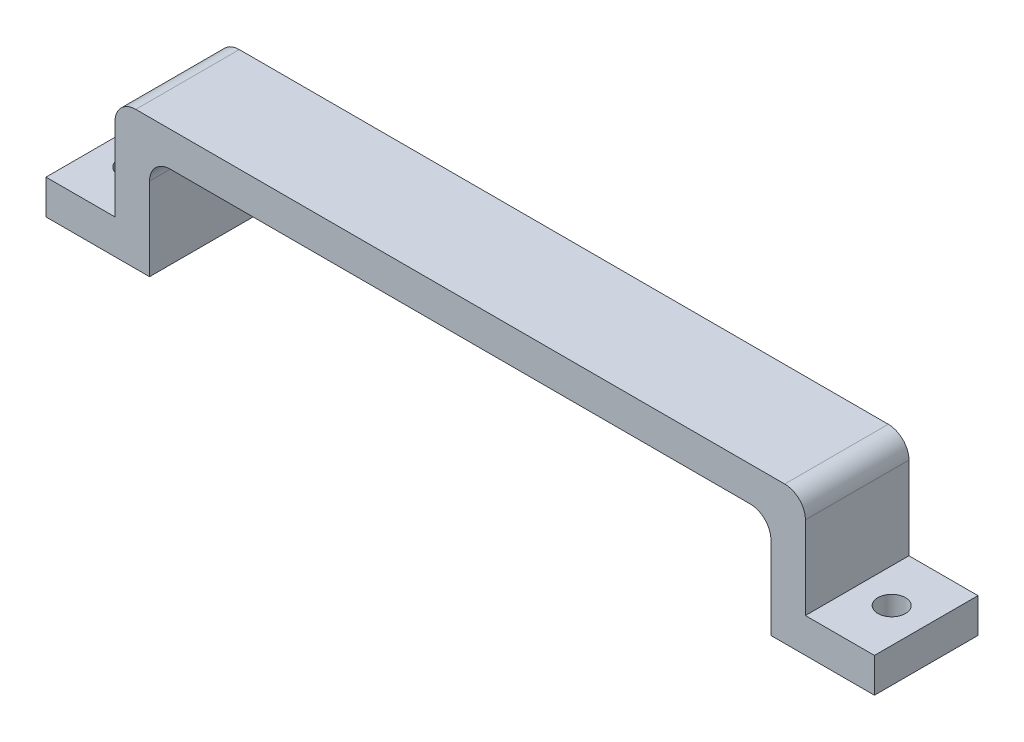
from build123d import *

# Parameters (mm, degrees)
EXTRUDE_1_DEPTH     = 15
SKETCH_2_R          = 2
CUT_EXTRUDE_1_DEPTH = 15
FILLET_1_R          = 3


with BuildPart() as part:
    # 草图1 → 凸台-拉伸1 (new body)
    with BuildSketch(Plane.XY):
        Polygon((0, 0), (15, 0), (15, 15), (105, 15), (105, 0), (120, 0), (120, 5), (110, 5), (110, 20), (10, 20), (10, 5), (0, 5), align=None)
    extrude(amount=EXTRUDE_1_DEPTH)

    # 草图2 → 切除-拉伸1 (cut)
    with BuildSketch(Plane(origin=(0, 5, 0), x_dir=(1, 0, 0), z_dir=(0, 1, 0))):
        with Locations(Location((5, -7.5, 0), (0, 0, 270))):
            Circle(SKETCH_2_R)
        with Locations(Location((115, -7.5, 0), (0, 0, 270))):
            Circle(SKETCH_2_R)
    extrude(amount=-CUT_EXTRUDE_1_DEPTH, mode=Mode.SUBTRACT)

    # 圆角1
    fillet_1_edges = [part.edges().sort_by_distance(p)[0] for p in [
        (10, 20, 7.5),
        (110, 20, 7.5),
        (105, 15, 7.5),
        (15, 15, 7.5),
    ]]
    fillet(fillet_1_edges, radius=FILLET_1_R)


solid = part.part
